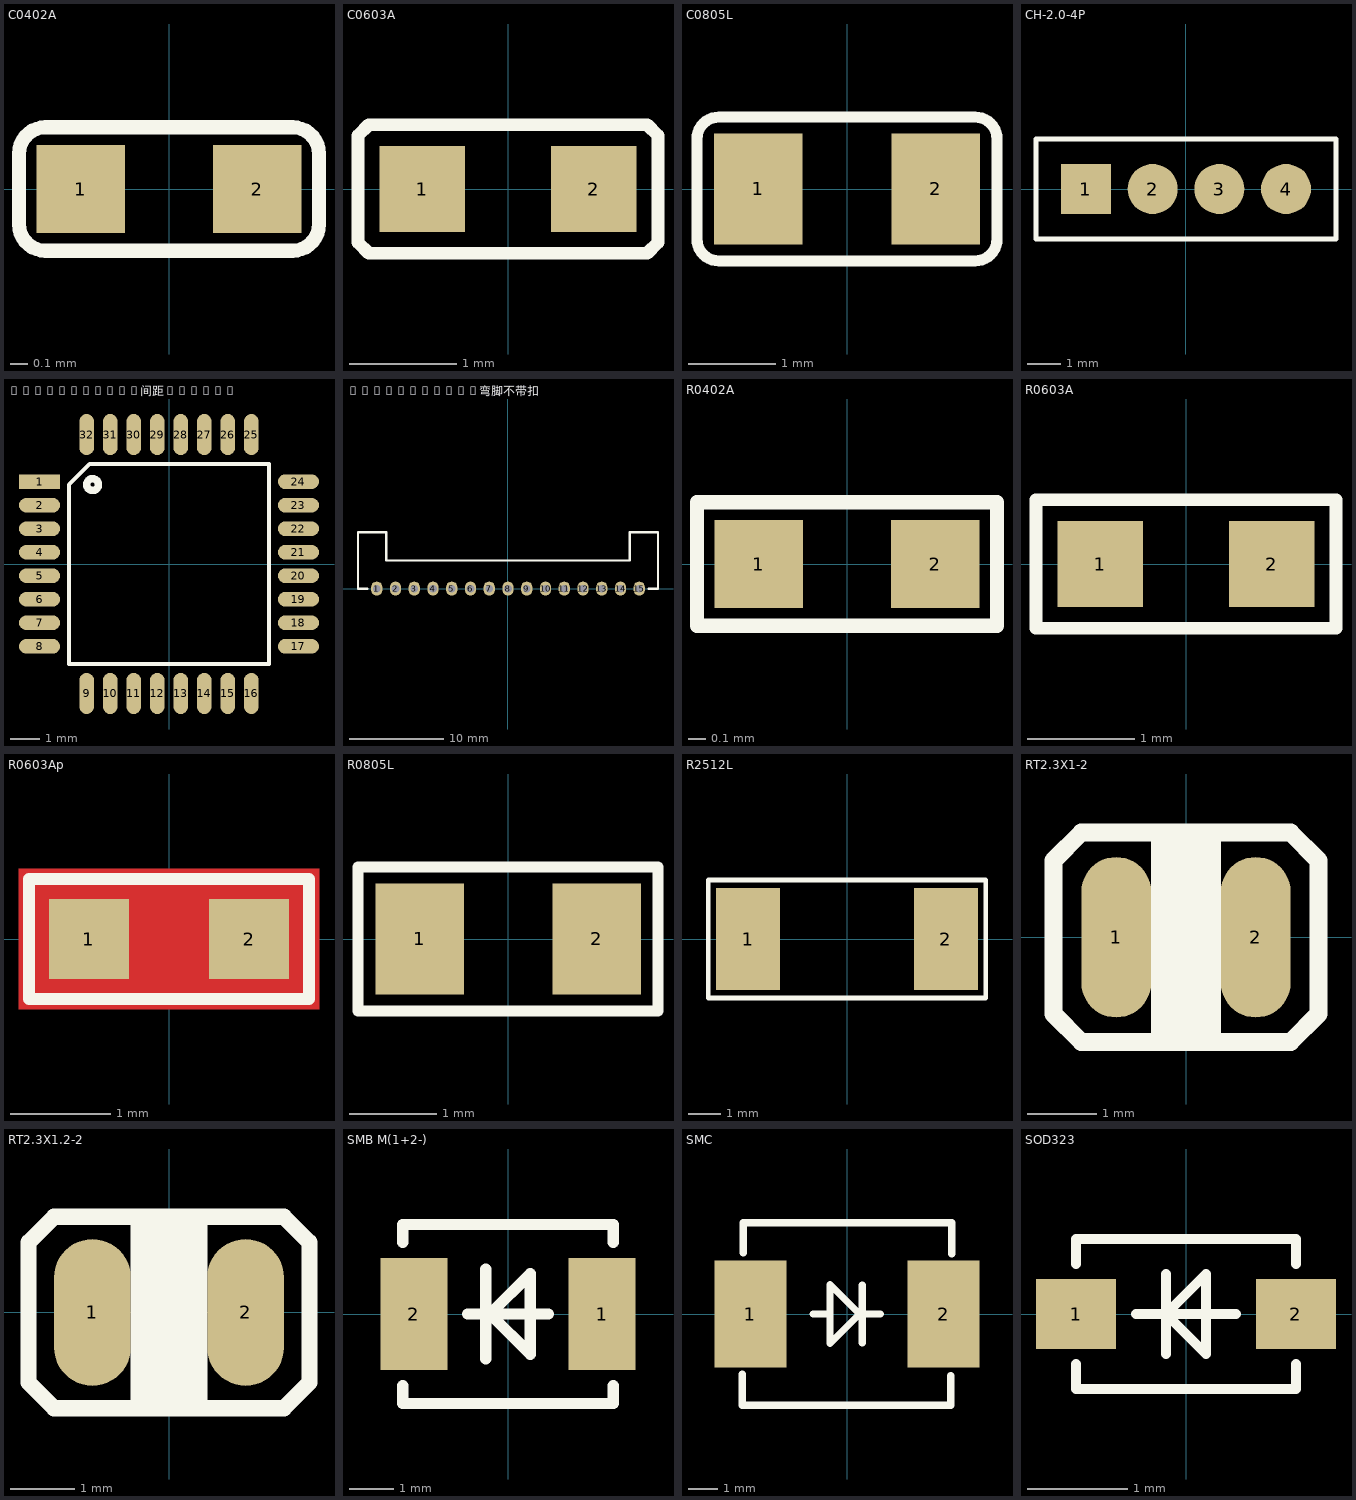
[diagram p0: the footprints below, top view; thin cyan lines are the x and y axes]
# Altium footprint library MISC84412-2.PcbLib: 22 footprints (part 1 of 2)
Each footprint in its own frame and in the unit in brackets; x right, y up, seen from the top. Pads: shape width x height; smd on the part's side, far side on the other; paste and mask are expansions set on the pad; w line width, h text height; cw(c..) or ccw(c..) is an arc to the next point about the centre after c.

## C0402A [mm] "SMD capacitor"
pads (2):
  rect 0.5x0.5 smd paste+0 mask+0.05: 1(-0.5,0) 2(0.5,0)
Top Overlay:
  lines w0.08: -0.85,-0.2 ccw(c-0.7,-0.2) -0.7,-0.35 0.7,-0.35 ccw(c0.7,-0.2) 0.85,-0.2 0.85,0.2 ccw(c0.7,0.2) 0.7,0.35 -0.7,0.35 ccw(c-0.7,0.2) -0.85,0.2 -0.85,-0.2

## C0603A [mm] "SMD capacitor"
pads (2):
  rect 0.8x0.8 smd mask+0.08: 1(-0.8,0) 2(0.8,0)
Top Overlay:
  lines w0.12: 0.551,-0.6 1.2,-0.6 ; -1.4,-0.5 -1.4,0.5 -1.3,0.6 1.3,0.6 1.4,0.5 1.4,-0.5 1.3,-0.6 -1.3,-0.6 -1.4,-0.5

## C0805L [mil] "SMD capacitor"
pads (2):
  rect 40x50 smd paste+0 mask+1.97: 1(-40,0) 2(40,0)
Top Overlay:
  lines w5: -67.72,-22.64 ccw(c-57.87,-22.64) -57.87,-32.48 57.87,-32.48 ccw(c57.87,-22.64) 67.72,-22.64 67.72,22.64 ccw(c57.87,22.64) 57.87,32.48 -57.87,32.48 ccw(c-57.87,22.64) -67.72,22.64 -67.72,-22.64

## CH-2.0-4P [mm] "Test socket 2.0mm"
pads (4):
  rect 1.5x1.5 smd: 1(-3,0)
  round 1.5 smd: 2(-1,0) 3(1,0) 4(3,0)
Top Overlay:
  lines w0.15: -4.5,-1.5 4.5,-1.5 4.5,1.5 -4.5,1.5 -4.5,-1.5

## LQFP32L(PIN间距0.8mm) [mm] "SMD IC (Sino Wealth SH3676014/16BP)"
height 3.35
pads (32):
  rect 1.4x0.5 smd: 1(-4.4,2.8)
  oval 1.4x0.5 smd: 2(-4.4,2) 3(-4.4,1.2) 4(-4.4,0.4) 5(-4.4,-0.4) 6(-4.4,-1.2) 7(-4.4,-2) 8(-4.4,-2.8) 17(4.4,-2.8) 18(4.4,-2) 19(4.4,-1.2) 20(4.4,-0.4) 21(4.4,0.4) 22(4.4,1.2) 23(4.4,2) 24(4.4,2.8)
  oval 0.5x1.4 smd: 9(-2.8,-4.4) 10(-2,-4.4) 11(-1.2,-4.4) 12(-0.4,-4.4) 13(0.4,-4.4) 14(1.2,-4.4) 15(2,-4.4) 16(2.8,-4.4) 25(2.8,4.4) 26(2,4.4) 27(1.2,4.4) 28(0.4,4.4) 29(-0.4,4.4) 30(-1.2,4.4) 31(-2,4.4) 32(-2.8,4.4)
Top Overlay:
  circle w0.254: c-2.6,2.7 r0.2
  lines w0.15: -3.4,-3.4 3.4,-3.4 3.4,3.4 -2.7,3.4 -3.4,2.7 -3.4,-3.4

## PH-2.0mm15P弯脚不带扣 [mm] "PH-2.0mm15P right-angle connector, no latch"
height 2.45
pads (15):
  oval 1.2x1.5 hole 0.8: 1(-14,0) 2(-12,0) 3(-10,0) 4(-8,0) 5(-6,0) 6(-4,0) 7(-2,0) 8(0,0) 9(2,0) 10(4,0) 11(6,0) 12(8,0) 13(10,0) 14(12,0) 15(14,0)
Top Overlay:
  lines w0.254: -15,0 -16,0 -16,6 -13,6 -13,3 13,3 13,6 16,6 16,0 15,0

## R0402A [mm] "SMD resistor"
pads (2):
  rect 0.5x0.5 smd paste+0 mask+0.05: 1(-0.5,0) 2(0.5,0)
Top Overlay:
  lines w0.08: -0.85,-0.35 0.85,-0.35 0.85,0.35 -0.85,0.35 -0.85,-0.35

## R0603A [mm] "SMD resistor"
height 0.5
pads (2):
  rect 0.8x0.8 smd mask+0.08: 1(-0.8,0) 2(0.8,0)
Top Overlay:
  lines w0.12: -1.4,-0.6 1.4,-0.6 1.4,0.6 -1.4,0.6 -1.4,-0.6

## R0603Ap [mm] "SMD resistor"
height 0.5
pads (2):
  rect 0.8x0.8 smd mask+0.08: 1(-0.8,0) 2(0.8,0)
Top Layer:
  pour cut-out: -1.5,0.7 1.5,0.7 1.5,-0.7 -1.5,-0.7
Top Overlay:
  lines w0.12: -1.4,-0.6 1.4,-0.6 1.4,0.6 -1.4,0.6 -1.4,-0.6

## R0805L [mil] "SMD resistor"
pads (2):
  rect 40x50 smd paste+0 mask+1.97: 1(-40,0) 2(40,0)
Top Overlay:
  lines w5: -67.91,-32.48 -67.91,32.48 ; -67.72,-32.48 67.72,-32.48 67.72,32.48 -67.72,32.48

## R2512L [mm] "SMD resistor"
pads (2):
  rect 2x3.2 smd: 1(-3.1,0) 2(3.1,0)
Top Overlay:
  lines w0.15: -4.35,-1.85 4.35,-1.85 4.35,1.85 -4.35,1.85 -4.35,-1.85

## RT2.3X1-2 [mm] "Wire-soldered NTC"
pads (2):
  oval 1x2.3 smd: 1(-1,0) 2(1,0)
Top Overlay:
  rectangle: -0.5,-1.55 0.5,1.5
  lines w0.254: -1.9,1.075 -1.9,-1.075 -1.9,-1.1 -1.5,-1.5 1.5,-1.5 1.9,-1.1 1.9,-1.075 1.9,1.075 ; -1.9,1.1 -1.5,1.5 1.5,1.5 1.9,1.1

## RT2.3X1.2-2 [mm] "Wire-soldered NTC"
height 2.45
pads (2):
  oval 1.2x2.3 smd: 1(-1.2,0) 2(1.2,0)
Top Overlay:
  rectangle: -0.6,-1.55 0.6,1.5
  lines w0.254: -2.2,-1.075 -2.2,1.075 ; -2.2,1.1 -1.8,1.5 ; 2.2,-1.075 2.2,1.075 ; 2.2,1.1 1.8,1.5 -1.8,1.5 ; -2.2,-1.1 -2.2,-1.1 ; -2.2,-1.1 -1.8,-1.5 ; -1.8,-1.5 1.8,-1.5 2.2,-1.1 ; -1.8,-1.5 -1.8,-1.5 ; -1.8,1.5 -1.8,1.5 ; 2.2,-1.1 2.2,-1.1

## SMB M(1+2-) [mm] "SMD diode"
pads (2):
  rect 1.5x2.5 smd: 1(2.1,0) 2(-2.1,0)
Top Overlay:
  lines w0.254: -2.35,-1.6 -2.35,-2 2.35,-2 2.35,-1.6 ; -2.35,1.6 -2.35,2 2.35,2 2.35,1.6 ; -0.9,0 0.9,0 ; -0.5,-1 -0.5,1 ; -0.4,0 0.5,0.9 0.5,-0.9 -0.4,0

## SMC [mm]
height 2.45
pads (2):
  rect 2.44x3.62 smd: 1(-3.275,0) 2(3.275,0)
Top Overlay:
  lines w0.25: -0.575,-1 0.425,0 -0.575,1 -0.575,-1
  lines w0.254: -3.55,-3.1 3.525,-3.1 3.525,-2.1 ; -3.55,-3.075 -3.55,-2.05 ; -3.525,2.075 -3.525,3.1 3.55,3.1 3.55,2.05 ; -1.15,0 -0.6,0 ; 0.5,0 1.125,0 ; 0.525,-0.975 0.525,0.025 ; 0.525,0 0.525,0.975

## SOD323 [mm] "SMD diode"
pads (2):
  rect 0.8x0.7 smd: 1(-1.1,0) 2(1.1,0)
Top Overlay:
  lines w0.1: -1.1,-0.5 -1.1,-0.75 1.1,-0.75 1.1,-0.5 ; -1.1,0.5 -1.1,0.75 1.1,0.75 1.1,0.5 ; -0.5,0 0.5,0 ; -0.2,-0.4 -0.2,0.4 ; -0.2,0 0.2,-0.4 0.2,0.4 -0.2,0